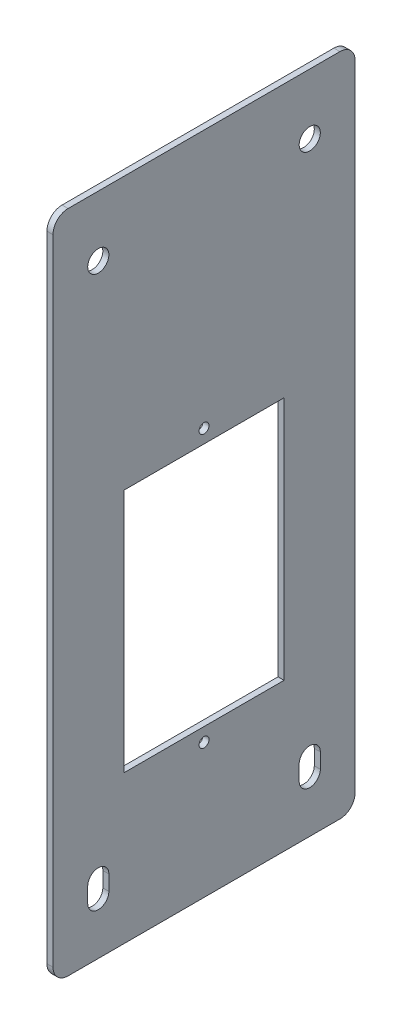
SolidWorks part; units mm, degrees
ref_plane "前视基准面" through (0, 0, 0) normal (0, 0, 1) x (1, 0, 0)
ref_plane "上视基准面" through (0, 0, 0) normal (0, 1, 0) x (1, 0, 0)
ref_plane "右视基准面" through (0, 0, 0) normal (1, 0, 0) x (0, 0, -1)
sketch "草图1" plane through (0, 0, 0) normal (0, 0, 1) x (1, 0, 0)
  line L0 (0, 220) -> (0, 0)
  line L1 (0, 0) -> (60, 0) construction
  dimension "D1" = 220
  dimension "D2" = 60
extrude "拉伸-薄壁1" add sketch "草图1" against normal blind 100 thin thin type one direction reverse wall 2
sketch "草图2" plane through (0, 0, 0) normal (-1, 0, 0) x (0, 0, 1)
  line L0 (-50, 220) -> (-50, 89.5) construction
  line L1 (-100, 220) -> (0, 220) construction
  line L2 (-100, 220) -> (0, 220) construction
  line L3 (-23.5, 130) -> (-76.5, 130)
  line L4 (-23.5, 130) -> (-23.5, 49)
  line L5 (-23.5, 49) -> (-76.5, 49)
  line L6 (-76.5, 130) -> (-76.5, 49)
  line L7 (-23.5, 130) -> (-76.5, 49) construction
  line L8 (-23.5, 49) -> (-76.5, 130) construction
  line L9 (-50, 89.5) -> (-50, 134.5) construction
  line L10 (-50, 89.5) -> (-50, 44.5) construction
  line L11 (-15, 200) -> (-85, 200) construction
  line L12 (-15, 200) -> (-15, 20) construction
  line L13 (-15, 20) -> (-85, 20) construction
  line L14 (-85, 200) -> (-85, 20) construction
  line L15 (-15, 200) -> (-85, 20) construction
  line L16 (-15, 20) -> (-85, 200) construction
  line L17 (-50, 89.5) -> (-50, 134.5) construction
  line L18 (-100, 0) -> (0, 0) construction
  line L19 (-15, 22.5) -> (-15, 17.5) construction
  line L20 (-11.5, 22.5) -> (-11.5, 17.5)
  line L21 (-18.5, 22.5) -> (-18.5, 17.5)
  line L22 (-85, 22.5) -> (-85, 17.5) construction
  line L23 (-81.5, 22.5) -> (-81.5, 17.5)
  line L24 (-88.5, 22.5) -> (-88.5, 17.5)
  circle A0 centre (-50, 44.5) radius 1.65
  circle A1 centre (-50, 134.5) radius 1.65
  circle A2 centre (-15, 200) radius 3.5
  circle A4 centre (-85, 200) radius 3.5
  arc A6 (-11.5, 22.5) -> (-18.5, 22.5) centre (-15, 22.5) ccw
  arc A7 (-18.5, 17.5) -> (-11.5, 17.5) centre (-15, 17.5) ccw
  arc A8 (-81.5, 22.5) -> (-88.5, 22.5) centre (-85, 22.5) ccw
  arc A9 (-88.5, 17.5) -> (-81.5, 17.5) centre (-85, 17.5) ccw
  point P12 (-50, 110)
  point P23 (-15, 20)
  point P31 (-85, 20)
  dimension "D5" = 3.3
  dimension "D9" = 7
  dimension "D4" = 90
  dimension "D1" = 81
  dimension "D2" = 53
  dimension "D3" = 90
  dimension "D6" = 20
  dimension "D7" = 20
  dimension "D8" = 70
  dimension "D10" = 7
  dimension "D11" = 5
extrude "切除-拉伸1" cut sketch "草图2" against normal blind 10
fillet "圆角1" radius 5 4 edges at (1, 220, -100) (1, 0, -100) (1, 0, 0) (1, 220, 0)
